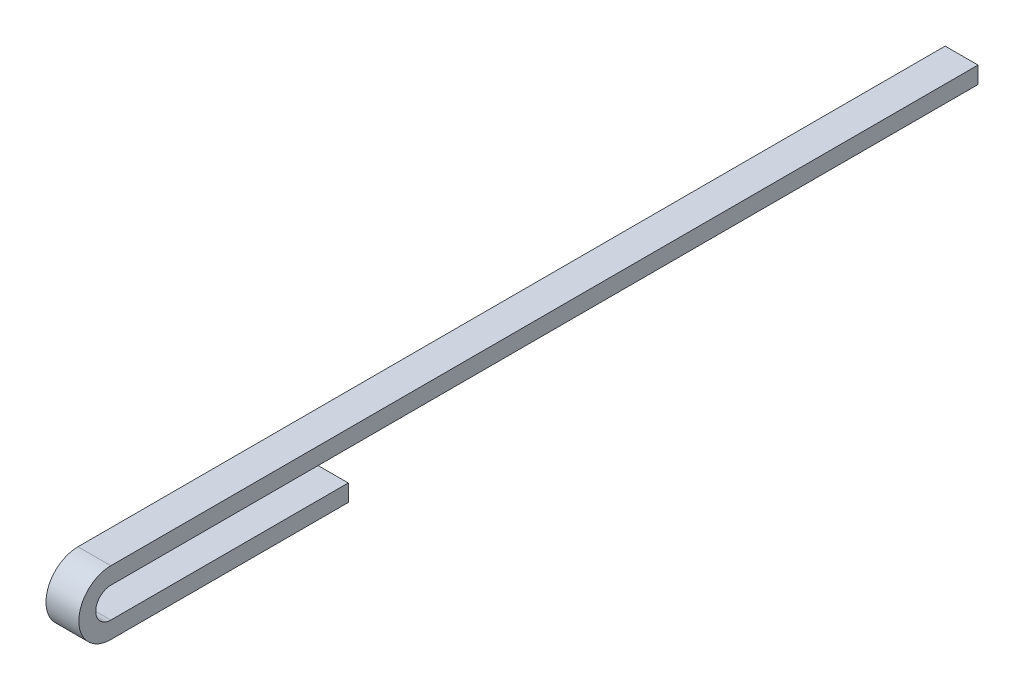
SolidWorks part; units mm, degrees
ref_plane "前视基准面" through (0, 0, 0) normal (0, 0, 1) x (1, 0, 0)
ref_plane "上视基准面" through (0, 0, 0) normal (0, 1, 0) x (1, 0, 0)
ref_plane "右视基准面" through (0, 0, 0) normal (1, 0, 0) x (0, 0, -1)
sketch "草图1" plane through (-86.9923, -141.23, -135.6926) normal (-1, 0, 0) x (0, 0, -1)
  line L0 (1100, 0) -> (-695.3148, 0)
  line L1 (1100, 0) -> (-1100, 0) construction
  line L2 (-203.7502, 132.4407) -> (-695.3148, 132.4407)
  line L3 (-203.7502, 97.4407) -> (-283.7502, 97.4407) construction
  arc A0 (-695.3148, 132.4407) -> (-695.3148, 0) centre (-695.3148, 66.2203) ccw
  dimension "D1" = 35
extrude "拉伸-薄壁1" add sketch "草图1" along normal mid plane 68 thin
